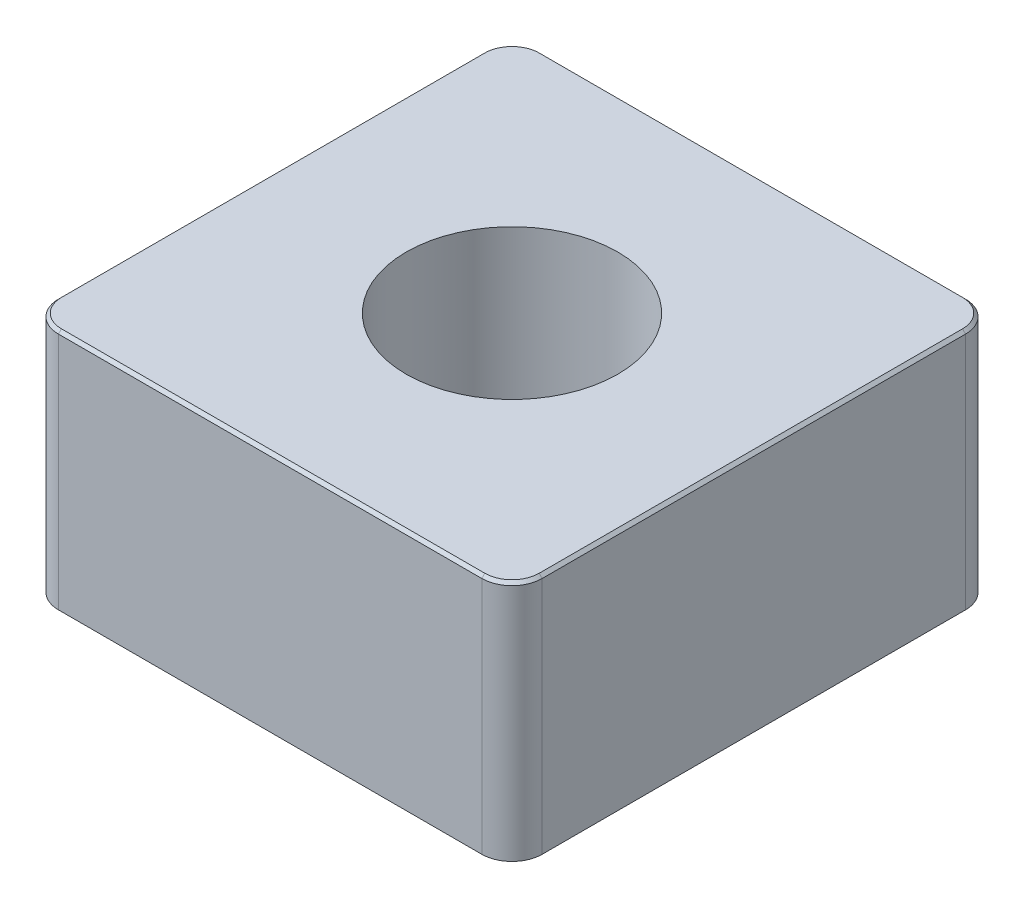
from build123d import *

# Parameters (mm, degrees)
SKETCH1_W             = 80
SKETCH1_H             = 80
BOSS_EXTRUDE1_DEPTH   = 40
M30_CLEARANCE_HOLE1_D = 35
FILLET1_R             = 5
CHAMFER1_SIZE         = 0.5


with BuildPart() as part:
    # Sketch1 → Boss-Extrude1 (new body)
    with BuildSketch(Plane(origin=(0, 15, 0), x_dir=(1, 0, 0), z_dir=(0, 1, 0))):
        Rectangle(SKETCH1_W, SKETCH1_H)
    extrude(amount=-BOSS_EXTRUDE1_DEPTH)

    # M30 Clearance Hole1 (through all)
    with Locations(Plane(origin=(0, 15, 0), x_dir=(1, 0, 0), z_dir=(0, 1, 0))):
        with Locations((0, 0)):
            Hole(M30_CLEARANCE_HOLE1_D / 2)

    # Fillet1
    fillet1_edges = [part.edges().sort_by_distance(p)[0] for p in [
        (-40, -5, -40),
        (40, -5, -40),
        (40, -5, 40),
        (-40, -5, 40),
    ]]
    fillet(fillet1_edges, radius=FILLET1_R)

    # Chamfer1
    chamfer1_edges = [part.edges().sort_by_distance(p)[0] for p in [
        (0, 15, 40),
        (-40, 15, 0),
        (40, 15, 0),
        (0, 15, -40),
        (-38.535533906, 15, -38.535533906),
        (38.535533906, 15, -38.535533906),
        (-38.535533906, 15, 38.535533906),
        (38.535533906, 15, 38.535533906),
    ]]
    chamfer(chamfer1_edges, length=CHAMFER1_SIZE)


solid = part.part
